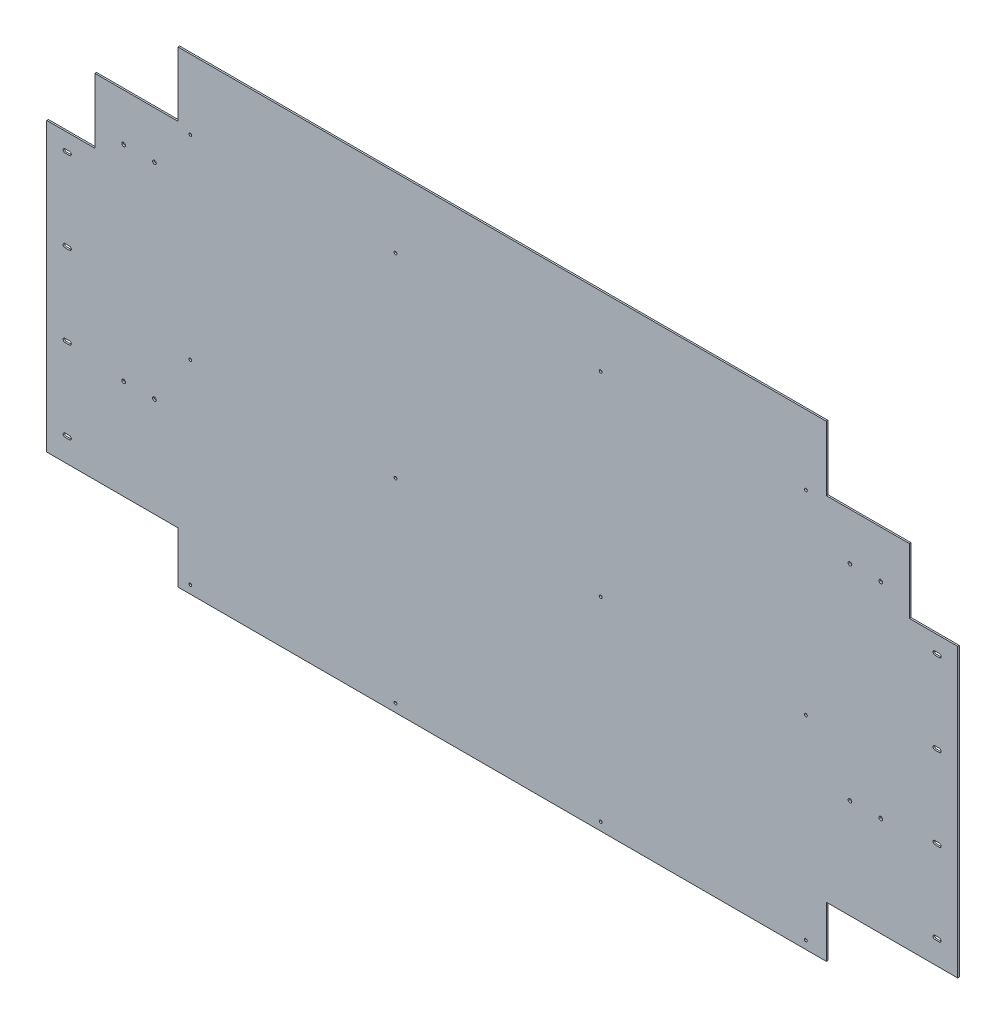
from build123d import *

# Parameters (mm, degrees)
BOSS_EXTRUDE1_DEPTH = 4
SKETCH2_R           = 3.5
SKETCH2_R_2         = 4.5
CUT_EXTRUDE1_DEPTH  = 4


with BuildPart() as part:
    # Sketch1 → Boss-Extrude1 (new body)
    with BuildSketch(Plane.XY):
        Polygon((-790, 570), (-790, 413), (-992.5, 413), (-992.5, 255), (-1110, 255), (-1110, -445), (-790, -445), (-790, -570), (790, -570), (790, -445), (1110, -445), (1110, 255), (992.5, 255), (992.5, 413), (790, 413), (790, 570), align=None)
    extrude(amount=BOSS_EXTRUDE1_DEPTH)

    # Sketch2 → Cut-Extrude1 (cut)
    with BuildSketch(Plane.XY.offset(4)):
        with Locations((-760, 400)):
            Circle(SKETCH2_R)
        with Locations((-260, 400)):
            Circle(SKETCH2_R)
        with Locations((240, 400)):
            Circle(SKETCH2_R)
        with Locations((740, 400)):
            Circle(SKETCH2_R)
        with Locations((-760, -75)):
            Circle(SKETCH2_R)
        with Locations((-260, -75)):
            Circle(SKETCH2_R)
        with Locations((240, -75)):
            Circle(SKETCH2_R)
        with Locations((740, -75)):
            Circle(SKETCH2_R)
        with Locations((-760, -550)):
            Circle(SKETCH2_R)
        with Locations((-260, -550)):
            Circle(SKETCH2_R)
        with Locations((240, -550)):
            Circle(SKETCH2_R)
        with Locations((740, -550)):
            Circle(SKETCH2_R)
        with Locations((-922.5, 298)):
            Circle(SKETCH2_R_2)
        with Locations((-847.5, 298)):
            Circle(SKETCH2_R_2)
        with Locations((-922.5, -202)):
            Circle(SKETCH2_R_2)
        with Locations((-847.5, -202)):
            Circle(SKETCH2_R_2)
        with Locations((847.5, 298)):
            Circle(SKETCH2_R_2)
        with Locations((922.5, 298)):
            Circle(SKETCH2_R_2)
        with Locations((847.5, -202)):
            Circle(SKETCH2_R_2)
        with Locations((922.5, -202)):
            Circle(SKETCH2_R_2)
        with BuildLine():
            Line((-1065.5, 217.5), (-1054.5, 217.5))
            ThreePointArc((-1054.5, 217.5), (-1050, 213), (-1054.5, 208.5))
            Line((-1054.5, 208.5), (-1065.5, 208.5))
            ThreePointArc((-1065.5, 208.5), (-1070, 213), (-1065.5, 217.5))
        make_face()
        with BuildLine():
            Line((-1065.5, 17.5), (-1054.5, 17.5))
            ThreePointArc((-1054.5, 17.5), (-1050, 13), (-1054.5, 8.5))
            Line((-1054.5, 8.5), (-1065.5, 8.5))
            ThreePointArc((-1065.5, 8.5), (-1070, 13), (-1065.5, 17.5))
        make_face()
        with BuildLine():
            Line((-1065.5, -182.5), (-1054.5, -182.5))
            ThreePointArc((-1054.5, -182.5), (-1050, -187), (-1054.5, -191.5))
            Line((-1054.5, -191.5), (-1065.5, -191.5))
            ThreePointArc((-1065.5, -191.5), (-1070, -187), (-1065.5, -182.5))
        make_face()
        with BuildLine():
            Line((-1065.5, -382.5), (-1054.5, -382.5))
            ThreePointArc((-1054.5, -382.5), (-1050, -387), (-1054.5, -391.5))
            Line((-1054.5, -391.5), (-1065.5, -391.5))
            ThreePointArc((-1065.5, -391.5), (-1070, -387), (-1065.5, -382.5))
        make_face()
        with BuildLine():
            Line((1065.5, -382.5), (1054.5, -382.5))
            ThreePointArc((1054.5, -382.5), (1050, -387), (1054.5, -391.5))
            Line((1054.5, -391.5), (1065.5, -391.5))
            ThreePointArc((1065.5, -391.5), (1070, -387), (1065.5, -382.5))
        make_face()
        with BuildLine():
            Line((1065.5, -182.5), (1054.5, -182.5))
            ThreePointArc((1054.5, -182.5), (1050, -187), (1054.5, -191.5))
            Line((1054.5, -191.5), (1065.5, -191.5))
            ThreePointArc((1065.5, -191.5), (1070, -187), (1065.5, -182.5))
        make_face()
        with BuildLine():
            Line((1065.5, 17.5), (1054.5, 17.5))
            ThreePointArc((1054.5, 17.5), (1050, 13), (1054.5, 8.5))
            Line((1054.5, 8.5), (1065.5, 8.5))
            ThreePointArc((1065.5, 8.5), (1070, 13), (1065.5, 17.5))
        make_face()
        with BuildLine():
            Line((1065.5, 217.5), (1054.5, 217.5))
            ThreePointArc((1054.5, 217.5), (1050, 213), (1054.5, 208.5))
            Line((1054.5, 208.5), (1065.5, 208.5))
            ThreePointArc((1065.5, 208.5), (1070, 213), (1065.5, 217.5))
        make_face()
    extrude(amount=-CUT_EXTRUDE1_DEPTH, mode=Mode.SUBTRACT)


solid = part.part
